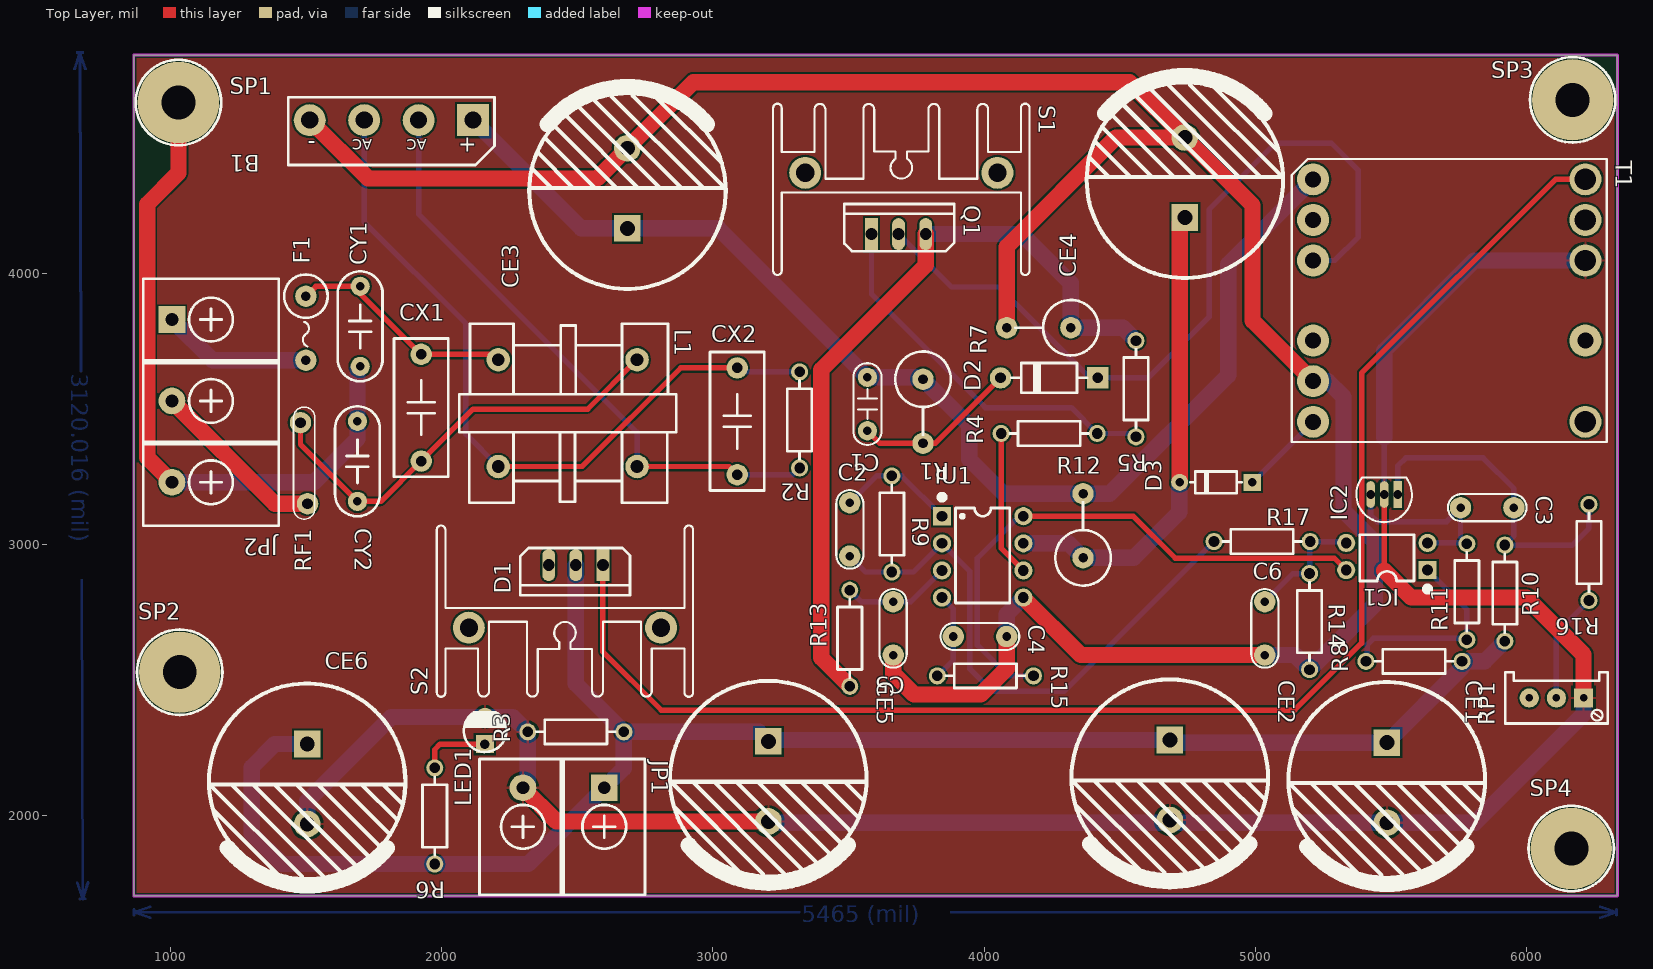
[diagram p0: Top Layer view]
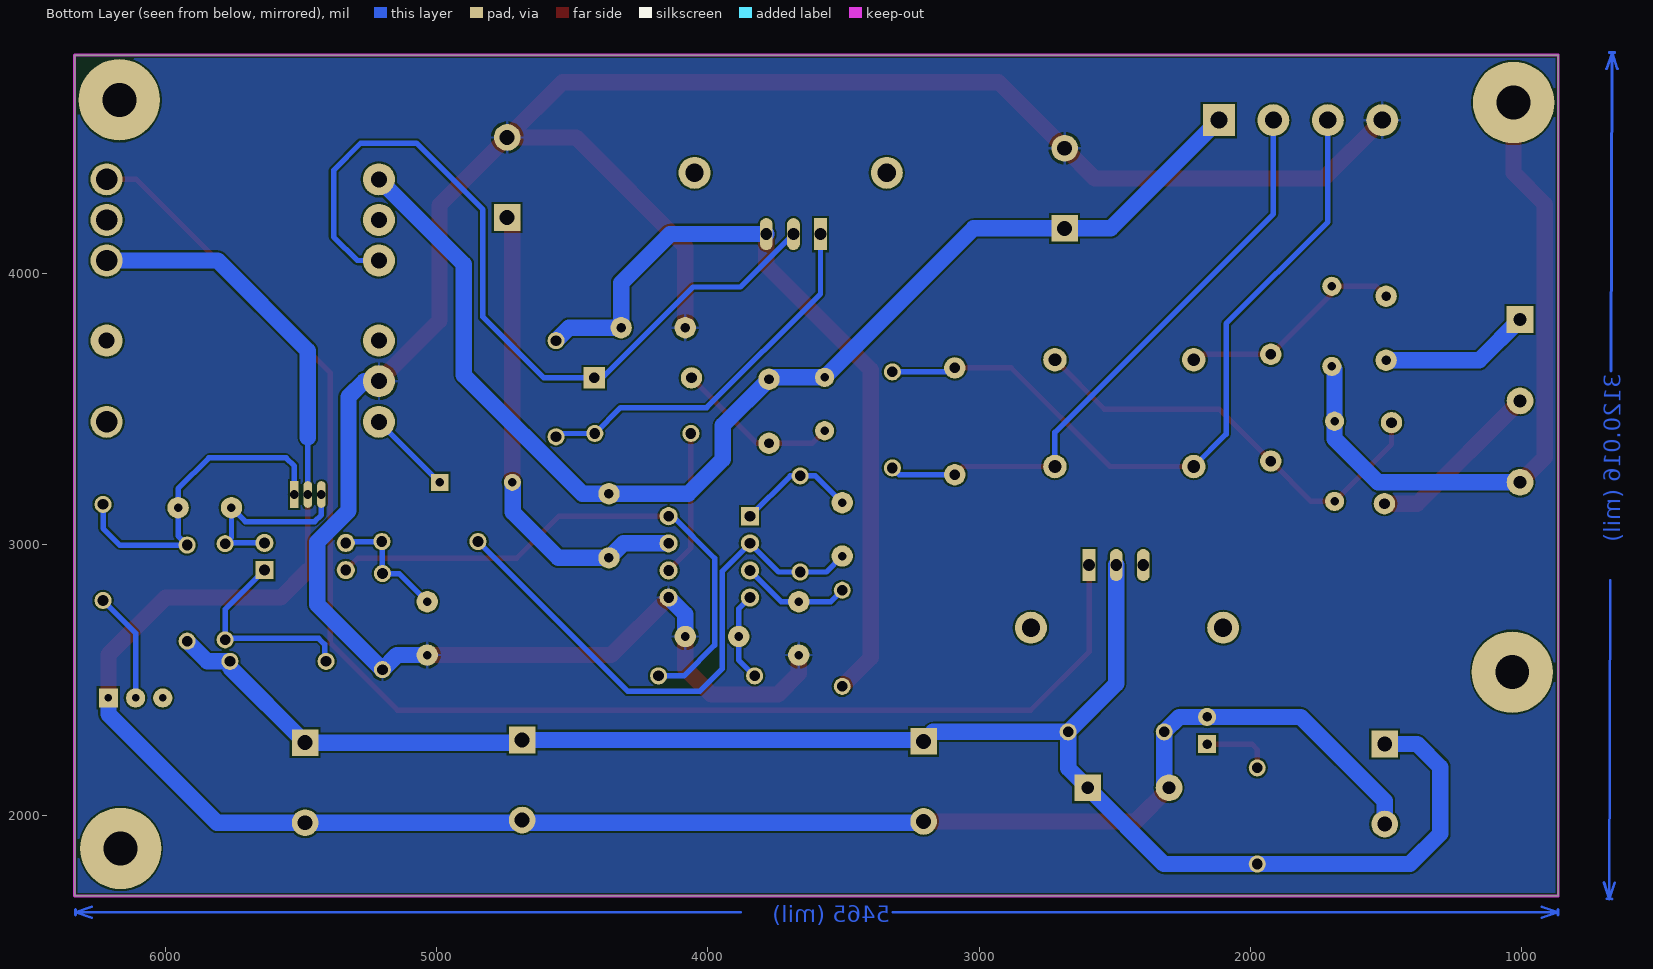
[diagram p1: Bottom Layer view, seen from below]
# Altium PCB MISC82119.PcbDoc
Units mil, origin at the board's own origin, x right, y up, seen from the top; angles counter-clockwise.
Board outline 5470 x 3100 mil, 2 copper layers (Top Layer, Bottom Layer); 55 components, 30 nets, 132 pads, 0 vias.

## Layer stack, top to bottom (the 12.6 mil dielectric is the usual default, probably not edited)
Top Solder: solder mask 0.4, Solder Resist, Dk 3.5
Top Layer: signal copper 1.4
Dielectric 1: dielectric 12.6, FR-4, Dk 4.8
Bottom Layer: signal copper 1.4
Bottom Solder: solder mask 0.4, Solder Resist, Dk 3.5

## Board outline
865,1705 865,4805 6335,4805 6335,1705

## Design rules (kind name [scope] priority, off if disabled: settings)
Clearance [All] p1: gap=7
Height [All] p1: minheight=0 maxheight=10000 prefheight=500
MinimumSolderMaskSliver [All] p1: minsoldermaskwidth=0
PolygonConnect [All] p1: connectstyle=Relief reliefconductorwidth=10 reliefentries=4 polygonreliefangle="90 Angle" airgapwidth=10
RoutingVias [All] p1: holewidth=28 width=50 viastyle="Through Hole" minholewidth=28 minwidth=50 maxholewidth=28 maxwidth=50
SilkToSilkClearance [All] p1: silktosilkclearance=0
SilkToSolderMaskClearance [IsPad] p1: minsilkscreentomaskgap=0 clearancetoexposedcopper=TRUE
SolderMaskExpansion [All] p1: expansion=4
Width [All] p1: maxlimit=100 minlimit=10 preferedwidth=10
26 further rules are at their usual default settings.

## Components (designator, comment, footprint, x,y, rotation, side; value= is the part's Value field where it differs from the comment)
B1 "KBL606" KBL 1815.39,4565 r180 top
C1 "330pF/1KV" "CY 5*7*2.5" 3570,3518.43 r270 top
C2 "10nF/50V" "CC 2*5" 3505,3056.5 r90 top
C3 "100nF/50V" "CC 2*5" 5855,3136.5 r0 top
C4 "2.2nF/50V" "CC 2*5" 3985,2661.5 r0 top
C5 "470pF/50V" "CC 2*5" 3665,2691.5 r270 top
C6 "1nF/50V" "CC 2*5" 5035,2691.5 r90 top
CE1 "470uF/35V" "CAP 7.5*18*35.5" 5485,2121.46 r270 top
CE2 "470uF/35V" "CAP 7.5*18*35.5" 4685,2131.46 r270 top
CE3 "120uF/450V" "CAP 7.5*18*35.5" 2685,4315 r90 top
CE4 "100uF/35V" "CAP 7.5*18*35.5" 4740,4355 r90 top
CE5 "470uF/35V" "CAP 7.5*18*35.5" 3205,2126.18 r270 top
CE6 "470uF/35V" "CAP 7.5*18*35.5" 1505,2116.46 r270 top
CX1 "0.1uF/275V" "CX 10-13*11" 1925,3505 r90 top
CX2 "0.1uF/275V" "CX 10-13*11" 3090,3455 r90 top
CY1 "1nF/250VAC" "CY 7.5*8*4" 1700,3805 r90 top
CY2 "1nF/250VAC" "CY 7.5*8*4" 1690,3307.36 r90 top
D1 "SBR20U100CT" TO220A 2495,2925 r180 top
D2 "FR107" DO-41 4240,3615 r180 top
D3 "1N4148" DO-35 4855,3230 r180 top
F1 "5x20/2A" "FU 4x16_V" 1500,3916.22 r270 top
IC1 "PC817" DIP4-300 5485,2956.5 r180 top
IC2 "TL431" TO92A 5475,3185 r90 top
IU1 "UC3842" DIP8-300 3995,2955 r0 top
JP1 "HDR-1X2" KF7620-2P 2450,1960 r180 top
JP2 "HDR-1X3" KF7620-3P 1150,3530 r270 top
L1 "20mH" UU10.5 2465,3485 r0 top
LED1 "Green" "LED 3MM-G" 2160,2315 r90 top
Q1 "IPA90R1K2C3" TO220A 3685,4145 r0 top
R1 "100K/2W" "RS 2W-V6" 3775,3610 r270 top
R2 "470K/0.25W" "RS 1/4W" 3320,3460 r270 top
R3 "1K/0.25W" "RS 1/4W" 2495,2310 r180 top
R4 "22Ω/0.25W" "RS 1/4W" 4240,3410 r180 top
R5 "10K/0.25W" "RS 1/4W" 4560,3575 r270 top
R6 "10K/0.25W" "RS 1/4W" 1975,2000 r270 top
R7 "0.2Ω/2W" "RS 2W-V6" 4320,3800 r180 top
R8 "270R/0.25W" "RS 1/4W" 5585,2570 r180 top
R9 "1K/0.25W" "RS 1/4W" 3660,3076.5 r270 top
R10 "20K/0.25W" "RS 1/4W" 5920,2821.5 r90 top
R11 "1K/0.25W" "RS 1/4W" 5780,2826.5 r90 top
R12 "100K/2W" "RS 2W-V6" 4365,2951.5 r90 top
R13 "1K/0.25W" "RS 1/4W" 3505,2655 r90 top
R14 "10K/0.25W" "RS 1/4W" 5200,2716.5 r270 top
R15 "8.87K/0.25W" "RS 1/4W" 4005,2516.5 r0 top
R16 "5.1K/0.25W" "RS 1/4W" 6230,2971.5 r270 top
R17 "1K/0.25W" "RS 1/4W" 5025,3011.5 r0 top
RF1 "5D-11" TVR-10D 1493,3157.4 r90 top
RP1 "500R" 3296W 6110,2435 r180 top
S1 "Heatsink" SRP16-24-25-P 3695,4310 r0 top
S2 "Heatsink" SRP16-24-25-P 2455,2755 r180 top
SP1 "M3 copper standoff" M3x4+6_N 1030,4630 r0 top
SP2 "M3 copper standoff" M3x4+6_N 1035,2530 r0 top
SP3 "M3 copper standoff" M3x4+6_N 6170,4640 r0 top
SP4 "M3 copper standoff" M3x4+6_N 6165,1880 r0 top
T1 "PQ2620" PQ2625+6PIN 5715,3900 r270 top

## Footprints (in the part's own frame and the unit in brackets; to place one, negate y for a bottom-side part, rotate by r counter-clockwise, add the part's x,y. Pads: shape width x height; smd on the part's side, far side on the other; paste and mask are expansions set on the pad)
3296W [mm] "Precise Multi-Winding Adjustable Resistor"
  rect 1.8x1.8 hole 0.7: 1(-2.54,0)
  round 1.8 hole 0.7: 2(0,0) 3(2.54,0)
  silkscreen extent -4.8,-2.4 4.8,2.4, body extent -4.75,-2.4 4.75,2.4, height 11.52
"CAP 7.5*18*35.5" [mm]
  rect 2.5x2.5 hole 1.4: 1(-3.78,0)
  round 2.5 hole 1.4: 2(3.72,0)
  silkscreen extent -9.44,-9.21 9.45,9.19, body extent -9,-9 9.01,9, height 35.54
"CC 2*5" [mm] "脚距2.2mm直径5mm"
  round 2 hole 0.8: 1(-2.5,0) 2(2.5,0)
  silkscreen extent -3.68,-1.27 3.68,1.27, body extent -2.4,-0.92 2.4,0.92, height 4.8
"CX 10-13*11" [mm]
  round 2 hole 1: 1(-5,0) 2(5,0)
  silkscreen extent -6.48,-2.54 6.48,2.54, body extent -6.5,-2.5 6.5,2.5, height 11.02
"CY 5*7*2.5" [mm]
  round 1.8 hole 0.8: 1(-2.5,0) 2(2.5,0)
  silkscreen extent -3.83,-1.31 3.83,1.31, body extent -3.5,-1.25 3.5,1.25, height 7
"CY 7.5*8*4" [mm] "脚距7.5mm，直径8mm，厚4mm"
  round 1.8 hole 0.8: 1(-3.75,0) 2(3.75,0)
  silkscreen extent -5.14,-2.1 5.14,2.1, body extent -4.04,-2 4.04,2, height 8.2
DIP4-300 [mm]
  rect 1.7x1.7 hole 1: 1(-3.81,1.27)
  round 1.7 hole 1: 2(-3.81,-1.27) 3(3.81,-1.27) 4(3.81,1.27)
  silkscreen extent -4.06,-2.03 2.54,3.3, body extent -3.93,-2.29 3.94,2.29, height 4.5
DIP8-300 [mm]
  rect 1.7x1.7 hole 1: 1(-3.81,3.81)
  round 1.7 hole 1: 2(-3.81,1.27) 3(-3.81,-1.27) 4(-3.81,-3.81) 5(3.81,-3.81) 6(3.81,-1.27) 7(3.81,1.27) 8(3.81,3.81)
  silkscreen extent -4.06,-4.32 2.54,5.84, body extent -3.93,-4.7 3.93,4.7, height 4.5
DO-35 [mm]
  rect 1.6x1.6 hole 0.8: 1(-3.4,0)
  round 1.6 hole 0.8: 2(3.4,0)
  silkscreen extent -2.41,-1.02 2.41,1.02, body extent -3.65,-0.9 3.65,0.9, height 1.85
DO-41 [mm]
  rect 2x2 hole 1: 1(-4.55,0)
  round 2 hole 1: 2(4.55,0)
  silkscreen extent -3.56,-1.4 3.56,1.4, body extent -4.92,-1.29 4.98,1.31, height 2.65
"FU 4x16_V" [mm]
  round 2 hole 0.9: 1(0,0) 2(6,0)
  silkscreen extent -2.03,-2.03 4.71,2.03, body extent -2,-2 6.3,2, height 13.1
KBL [mm]
  round 3 hole 1.6: AC1(2.55,0) AC2(-2.55,0) DC-(7.65,0)
  rect 3x3 hole 1.6: DC+(-7.65,0)
  silkscreen extent -9.65,-2.16 9.65,4.19, body extent -9.5,-2.1 9.5,4.15, height 14.21
KF7620-2P [mm] "15.2*12*12mm(长宽高)"
  rect 2.5x2.5 hole 1.2: 1(-3.81,-3.65)
  round 2.5 hole 1.2: 2(3.81,-3.65)
  silkscreen extent -7.62,-6.35 7.87,6.35, body extent -7.62,-6.2 8.32,6.2, height 12.45
KF7620-3P [mm] "22.8*12*12mm(长宽高)"
  rect 2.5x2.5 hole 1.2: 1(-7.62,-3.65)
  round 2.5 hole 1.2: 2(0,-3.65) 3(7.62,-3.65)
  silkscreen extent -11.43,-6.35 11.68,6.35, body extent -11.43,-6.2 12.13,6.2, height 12.45
"LED 3MM-G" [mm]
  rect 1.7x1.7 hole 0.9: 1(-1.27,0)
  round 1.7 hole 0.9: 2(1.27,0)
  silkscreen extent -2.01,-2 1.72,1.98, body extent -1.95,-1.95 1.64,1.95, height 5.55
M3x4+6_N [mil]
  round 300 hole 125: 1(0,0)
  silkscreen extent -157,-157 157,157, body extent -106,-93 106,93, height 159
PQ2625+6PIN [mm]
  round 3 hole 1.5: 1(-11.35,-12.75) 2(-7.55,-12.75) 3(-3.75,-12.75) 4(3.75,-12.75) 5(7.55,-12.75) 6(11.35,-12.75) 9(3.75,12.75)
  round 3 hole 2: 7(11.35,12.75) 10(-3.75,12.75) 11(-7.55,12.75) 12(-11.35,12.75)
  silkscreen extent -13.25,-14.75 13.25,14.75
"RS 1/4W" [mm]
  round 1.6 hole 1: 1(-4.5,0) 2(4.5,0)
  silkscreen extent -3.68,-1.14 3.68,1.14, body extent -4.72,-1.16 4.73,1.16, height 2.32
"RS 2W-V6" [mm]
  round 2 hole 0.9: 1(6,0) 2(0,0)
  silkscreen extent -2.6,-2.6 5.2,2.6, body extent -2.51,-2.51 6.4,2.51, height 17.6
SRP16-24-25-P [mm] "16mm*24mm*25mm(长*宽*高)"
  round 3 hole 1.7 unplated: 0(-9,1.55) 0(9,1.55)
  silkscreen extent -12,-8.02 12,8.02, body extent -12,-8 12,8, height 25.05
TO92A [mm]
  rect 2.5x0.8 hole 0.8: 1(0,-1.27)
  oval 2.5x0.8 hole 0.8: 2(0,0) 3(0,1.27)
  silkscreen extent -2.6,-2.6 1.6,2.6, body extent -2.3,-2.3 1.3,2.3, height 7.6
TO220A [mm]
  rect 1.2x3 hole 1.1: 1(-2.54,0)
  oval 1.2x3 hole 1.1: 2(0,0) 3(2.54,0)
  silkscreen extent -5.08,-1.6 5.21,2.82, body extent -5.15,-1.53 5.15,2.9, height 18.5
TVR-10D [mm]
  round 2 hole 1: 1(-0.159,-0.334) 2(7.432,0.33)
  silkscreen extent -1.61,-1.02 8.88,0.98, body extent -1.87,-0.93 9.42,0.92, height 16.5
UU10.5 [mm]
  round 2.2 hole 1.2: 1(-6.5,-5) 2(-6.5,5) 3(6.5,5) 4(6.5,-5)
  silkscreen extent -10.16,-8.38 10.16,8.38, body extent -9.4,-8 9.4,8, height 21.05

## Part data
B1: library part KBL, "600V/8A bridge rectifier"
C1 C2 C3 C4 C5 C6: library part CC, "Ceramic disc capacitor"
CE1 CE2 CE3 CE4 CE5 CE6: library part CE, "Through-hole electrolytic capacitor"
CX1 CX2: library part CX, "Safety X capacitor"
CY1 CY2: library part CY, "Safety Y capacitor"
D1 D2 D3: library part 1N4007, "Rectifier diode"
F1: library part "FU DIP", "Through-hole fuse"
IC1: library part 817, "Linear optocoupler"
IC2: library part TL431-ID, "Adjustable precision shunt regulator"
JP1: library part "Header 2", "2P connector"
JP2: library part "Header 3", "3P connector"
L1: library part L-UU, "Common-mode choke"
LED1: library part LED-3MM, "Through-hole 3mm LED"
Q1: library part IRF840, "N-channel MOSFET"
R1 R2 R3 R4 R5 R6 R7 R8 R9 R10 R11 R12 R13 R14 R15 R16 R17: library part R-S, "Color-band resistor"
RF1: library part PPTC, "PPTC resettable fuse"
RP1: library part RP, "Single-gang potentiometer"
S1 S2: library part S1
SP1 SP2 SP3 SP4: library part 铜柱加头大焊盘, "Copper standoff"
T1: "12V high-frequency transformer"

## Nets (pads, with @x,y where several pads share a name; then routed paths per layer and width w, separated by ;. In a path a pad name is that pad's centre, name@x,y a point inside that pad or via, vN(x,y) a via of type N, cw(c..) or ccw(c..) an arc to the next point about the centre after c; other vN are vias at no path point)
ACL: F1.2 JP2.1 | length 555.8
  Bottom Layer w60: JP2.1 1156.3,3680 F1.2
ACN: JP2.2 RF1.1 | length 656.8
  Top Layer w60: JP2.2 1385.16,3151.14 RF1.1
FB: C2.1 IU1.2 R9.2 R17.1 | length 2076
  Bottom Layer w20: C2.1 3563.74,2899.33 R9.2 3739.33,2899.33 IU1.2 3948,2902 3948,2542 4030,2460 4296.33,2460 R17.1
IS: Q1.3 R5.1 R7.2 R13.1 | length 2904.5
  Top Layer w60: R13.1 3400,2582.83 3400,3645 3785,4030 Q1.3
  Bottom Layer w60: Q1.3 4140,4145 4320,3965 R7.2 4512.17,3800 R5.1
NetB1_AC1: B1.AC1 CX2.2 L1.1 R2.1 | length 2749.1
  Top Layer w20: L1.1 2518.15,3288.15 2881.85,3651.85 CX2.2
  Bottom Layer w20: B1.AC1 1715,4190 2090,3815 2090,3407.24 L1.1 ; CX2.2 3104.68,3637.17 R2.1
NetB1_AC2: B1.AC2 CX2.1 L1.4 R2.2 | length 2232.1
  Top Layer w20: L1.4 3060,3288.15 CX2.1
  Bottom Layer w20: B1.AC2 1915.79,4219.21 2720.91,3414.09 L1.4 ; CX2.1 3295.32,3258.15 R2.2
NetC1_2: C1.2 D2.2 R1.1 | length 609.9
  Top Layer w20: C1.2 3616.22,3373.78 R1.1 3819.65,3373.78 D2.2
NetC2_2: C2.2 IU1.1 R9.1 | length 442.5
  Bottom Layer w20: C2.2 3603.74,3253.67 R9.1 3696.33,3253.67 IU1.1
NetC3_1: C3.1 IC1.2 IC2.3 R11.2 | length 723
  Bottom Layer w20: IC2.3 5425,3110 5450,3085 5705.07,3085 C3.1 5756.57,3027.09 R11.2@5777.17,3006.5 ; IC1.2 R11.2@5777.17,3006.5 ; R11.2 R11.2@5777.17,3006.5
NetC3_2: C3.2 IC2.1 R10.2 R16.1 | length 1238.7
  Bottom Layer w20: IC2.1 5525,3290 5555,3320 5840,3320 5953.43,3206.57 C3.2 5953.43,3032.09 R10.2 6168.67,2998.67 6230,3060 R16.1
NetC4_1: C4.1 IU1.4 R15.1 | length 330.1
  Bottom Layer w20: R15.1 3886.57,2575.24 C4.1 3886.57,2763.43 IU1.4
NetC5_1: C5.1 IU1.3 R13.2 | length 405.2
  Bottom Layer w20: R13.2 3547.24,2789.93 C5.1 3729.93,2789.93 IU1.3
NetC6_2: C6.2 IC1.3 R14.1 R17.2 | length 461.6
  Bottom Layer w20: C6.2 5138.74,2893.67 R14.1 5200,3009.33 R17.2 5330,3011.5 IC1.3
NetCX1_1: CX1.1 CY2.1 L1.3 RF1.2 | length 1624.4
  Top Layer w20: RF1.2 1480,3369.72 CY2.1 1776.57,3159.72 CX1.1 2116.85,3500 2539.06,3500 L1.3
NetCX1_2: CX1.2 CY1.2 F1.1 L1.2 | length 851.4
  Top Layer w20: F1.1 1536.42,3952.64 CY1.2 1700,3926.85 CX1.2 2189.09,3701.85 L1.2
NetD1_1: D1.1 T1.12 | length 5424.4
  Top Layer w20: D1.1 2595,2605 2810,2390 5145,2390 5392.25,2637.25 5392.25,3632.25 6106.85,4346.85 T1.12
NetD2_1: D2.1 Q1.2 T1.3 | length 2993.8
  Bottom Layer w20: Q1.2 3880,3950 4055,3950 4390,3615 D2.1 4605,3615 4830,3840 4830,4235 5075,4480 5280,4480 5380,4380 5380,4135 5292.64,4047.64 T1.3
NetD3_1: D3.1 T1.6 | length 316.6
  Bottom Layer w20: D3.1 5212.01,3453.15 T1.6
NetIC1_1: IC1.1 R8.2 R11.1 | length 760.8
  Bottom Layer w20: R8.2 5412.83,2575 5412.83,2632.83 5435,2655 5774.33,2655 R11.1 5780,2761.5 IC1.1
NetLED1_1: LED1.1 R6.1 | length 261.1
  Top Layer w20: R6.1 1975,2245 1995,2265 LED1.1
NetQ1_1: Q1.1 R4.1 R5.2 | length 1413.4
  Bottom Layer w20: Q1.1 3585,3925 4005,3505 4322.17,3505 R4.1 4547.83,3410 R5.2
NetR16_2: R16.2 RP1.2 | length 409
  Bottom Layer w20: RP1.2 6110,2674.33 R16.2
PE: CY1.1 CY2.2 JP2.3 SP1.1 | length 2506.9
  Top Layer w60: JP2.3 915,3321.3 915,4255 1030,4370 SP1.1
  Bottom Layer w60: JP2.3 1530,3230 1690,3390 CY2.2 1690,3647.36 CY1.1
PGND: B1.DC- C4.2 C5.2 C6.1 CE3.2 CE4.2 IU1.5 R7.1 R14.2 T1.5 | length 9061.3
  Top Layer w60: B1.DC- 1729.21,4350 2573.54,4350 CE3.2 2928.54,4705 4536.46,4705 CE4.2 ; C5.2 3665,2525 3742,2448 3988,2448 4083.43,2543.43 C4.2 ; R7.1 4083.78,4098.78 4486.46,4501.46 CE4.2 ; IU1.5 4356.93,2593.07 C6.1 ; T1.5 4990,3825.79 4990,4251.46 CE4.2
  Bottom Layer w60: C4.2 4083.43,2743.43 IU1.5 ; C6.1 5146.26,2593.07 R14.2 5440,2779.33 5440,3010 5325,3125 5325,3545 5267.24,3602.76 T1.5
PWM: IU1.6 R4.2 | length 539
  Top Layer w20: R4.2 4062.83,2987.17 IU1.6
SGND: CE1.2 CE2.2 CE5.2 CE6.2 IC2.2 JP1.2 LED1.2 R3.2 RP1.1 T1.10 | length 8164.9
  Top Layer w20: 5475,2905 IC2.2
  Top Layer w60: JP1.2 2423.98,1979.72 CE5.2 ; 5475,2905 5575,2805 6000,2805 6210,2595 RP1.1
  Bottom Layer w20: IC2.2 5475,3395
  Bottom Layer w60: CE6.2 1505,2055 1815,2365 LED1.2 2262.83,2365 R3.2 2317.83,2121.54 JP1.2 ; CE5.2 3209.72,1975 CE1.2 5810,1975 6210,2375 RP1.1 ; 5475,3395 5475,3715 5807.64,4047.64 T1.10
VBUS: B1.DC+ C1.1 CE3.1 R1.2 R12.1 T1.1 | length 4459.8
  Bottom Layer w60: B1.DC+ 2515.39,4166.18 CE3.1 3020.67,4166.18 C1.1 3768.15,3616.85 R1.2 3945,3440 3945,3315 4072.28,3187.72 R12.1 4462.72,3187.72 4900,3625 4900,4033.82 T1.1
VCC: CE4.1 D3.2 IU1.7 R12.2 | length 1761.4
  Top Layer w60: D3.2 4721.14,4187.32 CE4.1
  Bottom Layer w60: IU1.7 4311.5,3005 R12.2 4551.5,2951.5 4720,3120 4720,3228.86 D3.2
VOUT: CE1.1 CE2.1 CE5.1 CE6.1 D1.2 JP1.1 R3.1 R6.2 R8.1 R10.1 | length 6309.5
  Bottom Layer w60: CE6.1 1385.28,2265.28 1300,2180 1300,1935 1412.17,1822.83 R6.2 2319.13,1822.83 JP1.1 2672.17,2175.87 R3.1 ; D1.2 2495,2487.17 R3.1 ; R10.1 5845.67,2570 R8.1 5762.17,2547.44 CE1.1 4695,2270.28 CE2.1 3210.28,2280.28 CE5.1 3170,2310 R3.1
VREF: IC1.4 IU1.8 R15.2 | length 2080.6
  Top Layer w20: IU1.8 4550,3105 4705,2950 5291.5,2950 IC1.4
  Bottom Layer w20: IU1.8 4130,3105 3975,2950 3975,2630 4088.5,2516.5 R15.2
pads on no net: D1.3 RP1.3 S1.0 S2.0 SP2.1 SP3.1 SP4.1 T1.2 T1.4 T1.7 T1.9 T1.11
copper on no net: | length 7837.4
  Bottom Layer w10: 647.16,4754.15 666.97,4814.21 ; 656.78,1754.15 676.97,1694.21 ; 656.97,4814.18 676.97,4814.25 ; 666.97,1694.18 686.97,1694.25 ; 670.73,3640.09 666.97,4814.21 ; 673.21,2868.34 676.97,1694.21 ; 687.16,4754.28 666.97,4814.21 ; 696.78,1754.28 676.97,1694.21 ; 866.6,1635 866.6,1655 ; 926.6,1625 866.6,1645 ; 926.6,1665 866.6,1645 ; 3318.19,1645 866.6,1645 ; 3880.02,1645 6331.6,1645 ; 6271.6,1625 6331.6,1645 ; 6271.6,1665 6331.6,1645 ; 6331.6,1635 6331.6,1655

## Polygon pours and split planes (outlines as drawn)
SGND on Top Layer "Top Layer-No Net" (solid, remove dead copper, pour order 6): 370,5405 470,5305 6910,5305 6910,1390 6550,1030 6290,1290 350,1290
PGND on Bottom Layer "Top Layer-No Net" (solid, remove dead copper, pour order 8): 415,5125 6765,5125 6880,5240 6635,4995 6635,855 800,855 435,1220

## Keep-outs
Keep-Out Layer:
  lines w10: 865,1705 6335,1705 6335,4805 865,4805 865,2340 865,1705

## Other copper
Bottom Layer:
  text "3120.016 (mil)" at 634.78,3629.98 h60 r270.18
  text "5465 (mil)" at 3328.19,1609.01 h60